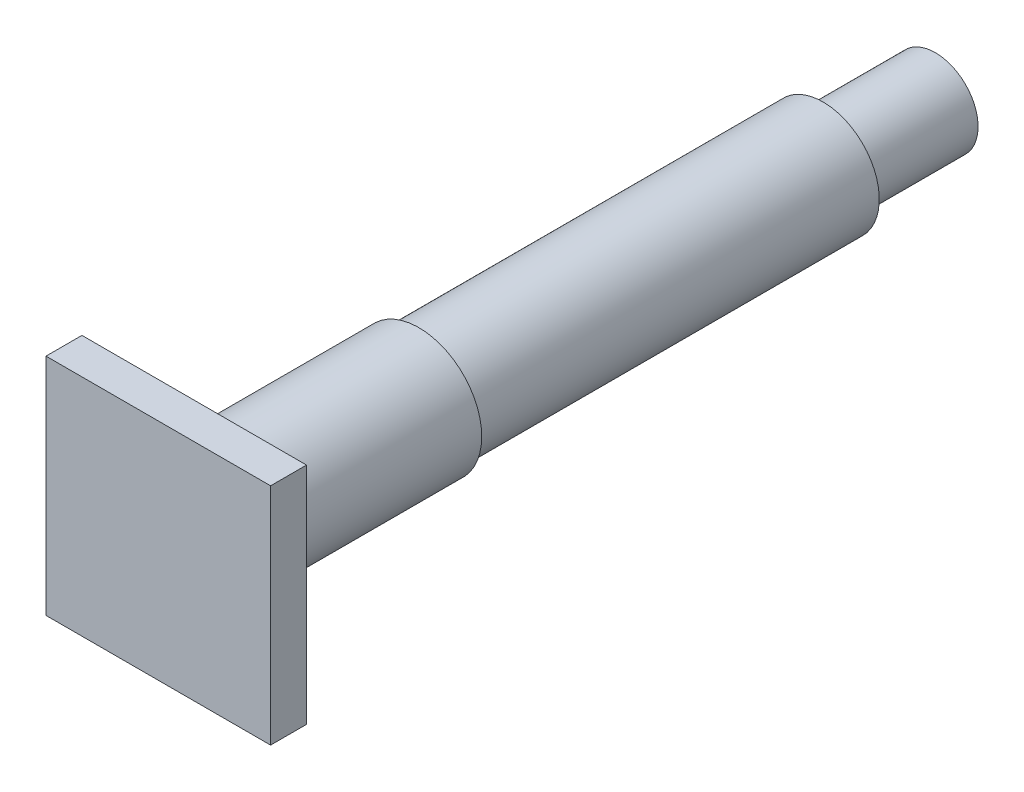
SolidWorks part; units mm, degrees
ref_plane "前视基准面" through (0, 0, 0) normal (0, 0, 1) x (1, 0, 0)
ref_plane "上视基准面" through (0, 0, 0) normal (0, 1, 0) x (1, 0, 0)
ref_plane "右视基准面" through (0, 0, 0) normal (1, 0, 0) x (0, 0, -1)
sketch "草图1" plane through (0, 0, 0) normal (0, 0, 1) x (1, 0, 0)
  circle A0 centre (0, 0) radius 12.5
  dimension "D1" = 25
extrude "凸台-拉伸1" add sketch "草图1" along normal blind 90
sketch "草图2" plane through (0, 0, 90) normal (0, 0, 1) x (1, 0, 0)
  circle A0 centre (0, 0) radius 14
  dimension "D1" = 28
extrude "凸台-拉伸2" add sketch "草图2" along normal blind 50
sketch "草图3" plane through (0, 0, 140) normal (0, 0, 1) x (1, 0, 0)
  line L1 (-25, -25) -> (25, -25)
  line L2 (-25, -25) -> (-25, 25)
  line L3 (-25, 25) -> (25, 25)
  line L4 (25, -25) -> (25, 25)
  line L5 (-25, -25) -> (25, 25) construction
  line L6 (-25, 25) -> (25, -25) construction
  point P0 (0, 0)
  dimension "D1" = 50
extrude "凸台-拉伸3" add sketch "草图3" along normal blind 8
sketch "草图4" plane through (0, 0, 0) normal (0, 0, -1) x (-1, 0, 0)
  circle A0 centre (0, 0) radius 9.5
  dimension "D1" = 19
extrude "凸台-拉伸4" add sketch "草图4" along normal blind 25
sketch "草图5" plane through (0, 0, -25) normal (0, 0, -1) x (-1, 0, 0)
  circle A0 centre (0, 0) radius 9.5
  dimension "D1" = 19
